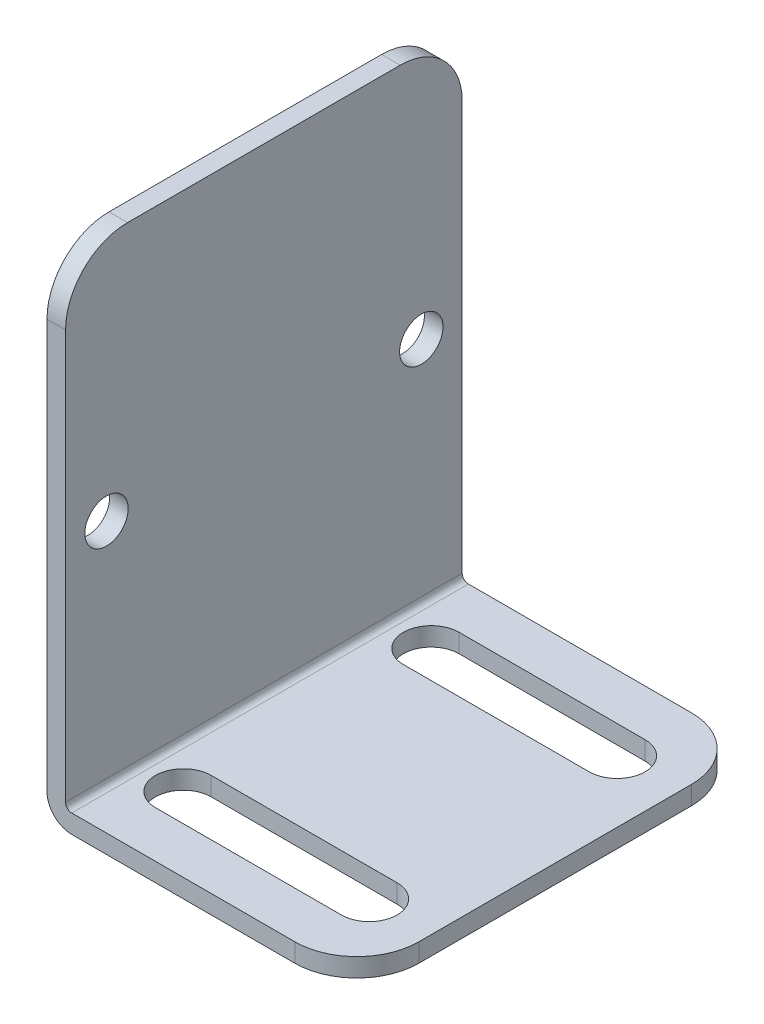
from build123d import *

# Parameters (mm, degrees)
EXTRUDE_1_DEPTH     = 32
FILLET_1_R          = 0.5
FILLET_2_R          = 2
FILLET_3_R          = 5
CUT_EXTRUDE_1_REACH = 59
SKETCH_2_R          = 1.75
CUT_EXTRUDE_2_REACH = 57.958


with BuildPart() as part:
    # 草图1 → 拉伸-薄壁1 (new body)
    with BuildSketch(Plane.XY):
        Polygon((25, 0), (0, 0), (0, 40), (1.5, 40), (1.5, 1.5), (25, 1.5), align=None)
    extrude(amount=EXTRUDE_1_DEPTH)

    # 圆角1
    fillet_1_edges = [part.edges().sort_by_distance(p)[0] for p in [
        (1.5, 1.5, 16),
    ]]
    fillet(fillet_1_edges, radius=FILLET_1_R)

    # 圆角2
    fillet_2_edges = [part.edges().sort_by_distance(p)[0] for p in [
        (0, 0, 16),
    ]]
    fillet(fillet_2_edges, radius=FILLET_2_R)

    # 圆角3
    fillet_3_edges = [part.edges().sort_by_distance(p)[0] for p in [
        (0.75, 40, 32),
        (0.75, 40, 0),
        (25, 0.75, 0),
        (25, 0.75, 32),
    ]]
    fillet(fillet_3_edges, radius=FILLET_3_R)

    # 草图2 → 切除-拉伸1 (cut, up to next)
    with BuildSketch(Plane.ZY, mode=Mode.PRIVATE) as cut_extrude_1_sk1:
        with Locations((3.3, 20)):
            Circle(SKETCH_2_R)
    cut_extrude_1_tool1 = extrude(cut_extrude_1_sk1.sketch, amount=-CUT_EXTRUDE_1_REACH, mode=Mode.PRIVATE) & part.part
    # 草图2 → 切除-拉伸1 (cut, up to next)
    with BuildSketch(Plane.ZY, mode=Mode.PRIVATE) as cut_extrude_1_sk2:
        with Locations((28.7, 20)):
            Circle(SKETCH_2_R)
    cut_extrude_1_tool2 = extrude(cut_extrude_1_sk2.sketch, amount=-CUT_EXTRUDE_1_REACH, mode=Mode.PRIVATE) & part.part
    add(cut_extrude_1_tool1.solids().sort_by_distance((0, 20, 3.3))[0], mode=Mode.SUBTRACT)
    add(cut_extrude_1_tool2.solids().sort_by_distance((0, 20, 28.7))[0], mode=Mode.SUBTRACT)

    # 草图3 → 切除-拉伸2 (cut, up to next)
    with BuildSketch(Plane(origin=(0, 1.5, 0), x_dir=(1, 0, 0), z_dir=(0, 1, 0)), mode=Mode.PRIVATE) as cut_extrude_2_sk1:
        with BuildLine():
            Line((5, -3.75), (20, -3.75))
            ThreePointArc((20, -3.75), (22.25, -6), (20, -8.25))
            Line((20, -8.25), (5, -8.25))
            ThreePointArc((5, -8.25), (2.75, -6), (5, -3.75))
        make_face()
    cut_extrude_2_tool1 = extrude(cut_extrude_2_sk1.sketch, amount=-CUT_EXTRUDE_2_REACH, mode=Mode.PRIVATE) & part.part
    # 草图3 → 切除-拉伸2 (cut, up to next)
    with BuildSketch(Plane(origin=(0, 1.5, 0), x_dir=(1, 0, 0), z_dir=(0, 1, 0)), mode=Mode.PRIVATE) as cut_extrude_2_sk2:
        with BuildLine():
            Line((5, -23.75), (20, -23.75))
            ThreePointArc((20, -23.75), (22.25, -26), (20, -28.25))
            Line((20, -28.25), (5, -28.25))
            ThreePointArc((5, -28.25), (2.75, -26), (5, -23.75))
        make_face()
    cut_extrude_2_tool2 = extrude(cut_extrude_2_sk2.sketch, amount=-CUT_EXTRUDE_2_REACH, mode=Mode.PRIVATE) & part.part
    add(cut_extrude_2_tool1.solids().sort_by_distance((12.5, 1.5, 6))[0], mode=Mode.SUBTRACT)
    add(cut_extrude_2_tool2.solids().sort_by_distance((12.5, 1.5, 26))[0], mode=Mode.SUBTRACT)


solid = part.part
